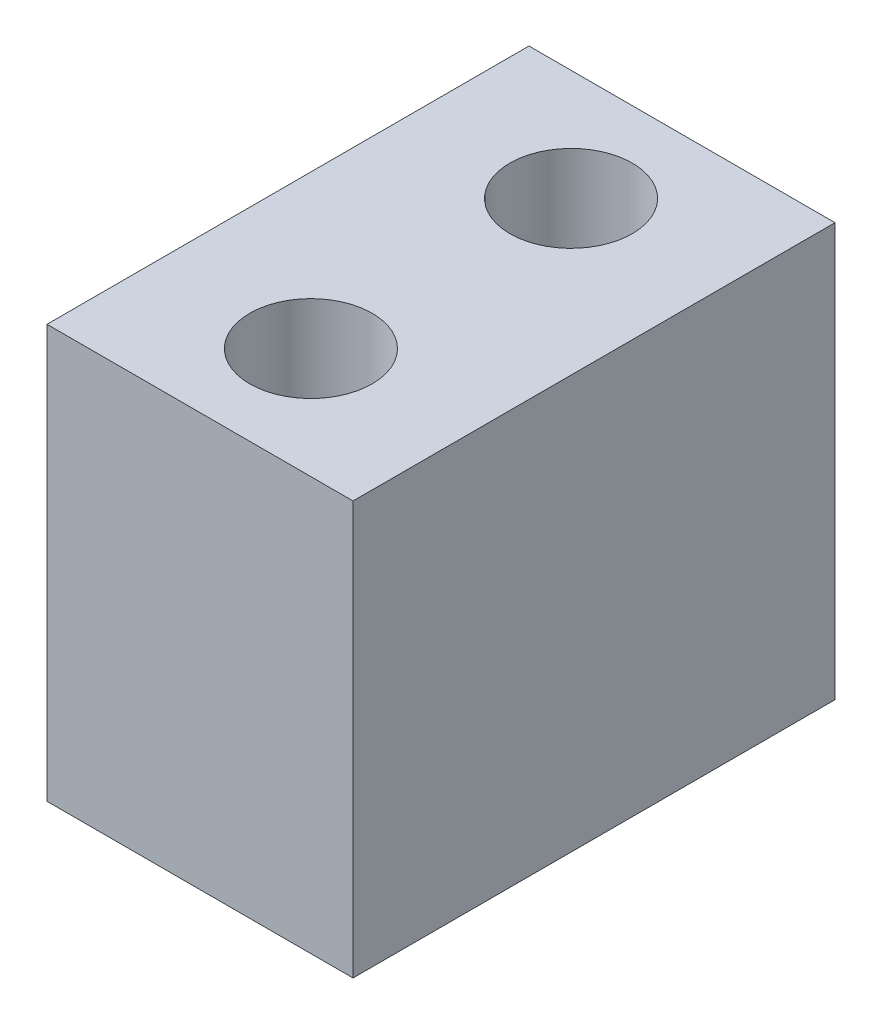
from build123d import *

# Parameters (mm, degrees)
SKETCH2_W              = 80
SKETCH2_H              = 126
BOSS_EXTRUDE1_DEPTH    = 54
M36_TAPPED_HOLE1_D     = 32
M36_TAPPED_HOLE1_DEPTH = 80
M36_TAPPED_HOLE1_TIP   = 9.613769904


with BuildPart() as part:
    # Sketch2 → Boss-Extrude1 (new, symmetric)
    with BuildSketch(Plane(origin=(0, 0, 0), x_dir=(1, 0, 0), z_dir=(0, 1, 0))):
        Rectangle(SKETCH2_W, SKETCH2_H)
    extrude(amount=BOSS_EXTRUDE1_DEPTH, both=True)

    # M36 Tapped Hole1
    with Locations(Plane(origin=(0, 54, 0), x_dir=(1, 0, 0), z_dir=(0, 1, 0))):
        with Locations((0, 34), (0, -34)):
            Hole(M36_TAPPED_HOLE1_D / 2, depth=M36_TAPPED_HOLE1_DEPTH)
            with Locations((0, 0, -(M36_TAPPED_HOLE1_DEPTH + M36_TAPPED_HOLE1_TIP / 2))):  # 118° drill point
                Cone(0, M36_TAPPED_HOLE1_D / 2, M36_TAPPED_HOLE1_TIP, mode=Mode.SUBTRACT)


solid = part.part
